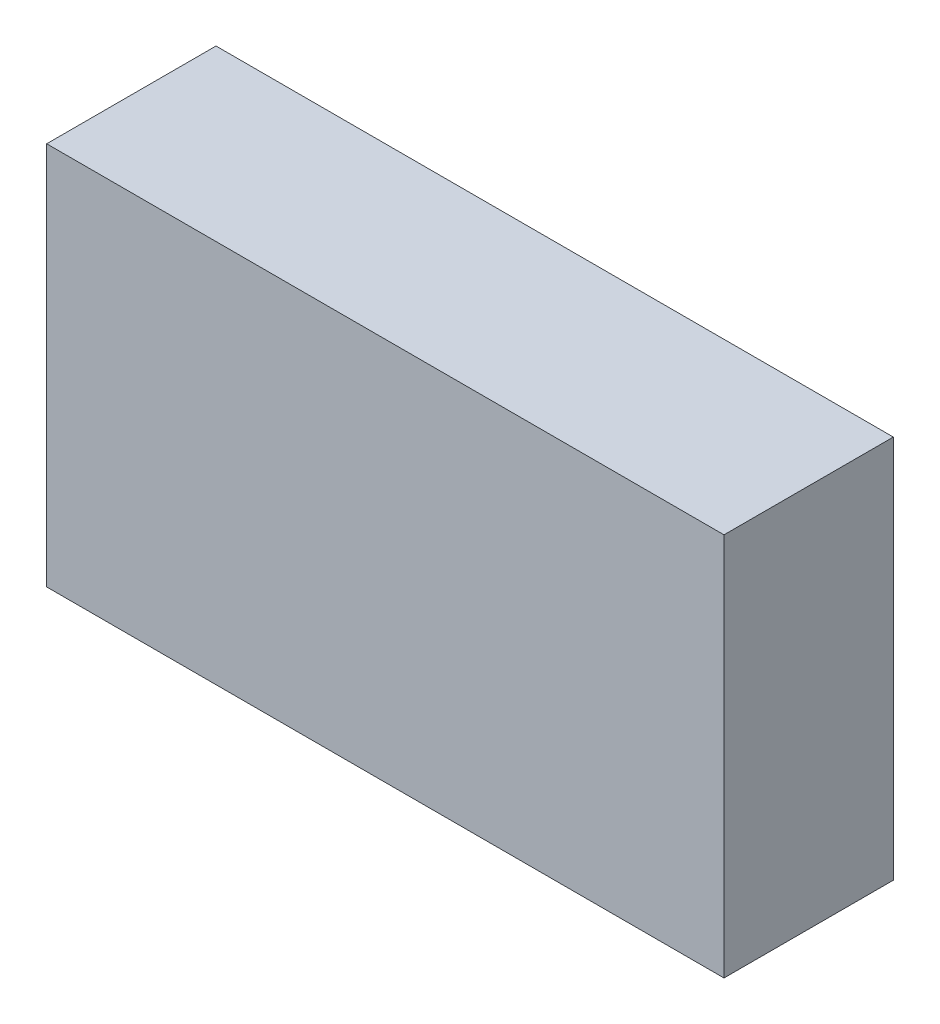
from build123d import *

# Parameters (mm, degrees)
SKETCH_1_W      = 60
SKETCH_1_H      = 34
EXTRUDE_1_DEPTH = 15


with BuildPart() as part:
    # 草图1 → 凸台-拉伸1 (new body)
    with BuildSketch(Plane.XY):
        Rectangle(SKETCH_1_W, SKETCH_1_H)
    extrude(amount=EXTRUDE_1_DEPTH)


solid = part.part
